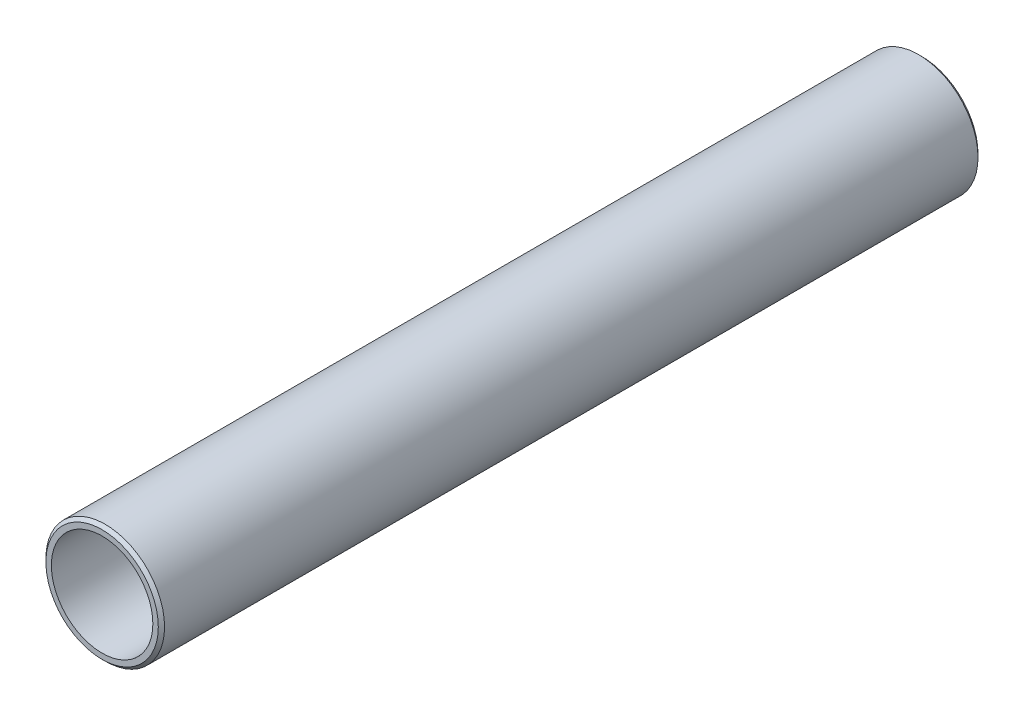
from build123d import *

# Parameters (mm, degrees)
SKETCH_1_R      = 38
SKETCH_1_R_2    = 32.5
EXTRUDE_1_DEPTH = 525
CHAMFER_1_SIZE  = 2


with BuildPart() as part:
    # 草图1 → 凸台-拉伸1 (new body)
    with BuildSketch(Plane.XY):
        Circle(SKETCH_1_R)
        Circle(SKETCH_1_R_2, mode=Mode.SUBTRACT)
    extrude(amount=EXTRUDE_1_DEPTH)

    # 倒角1
    chamfer_1_edges = [part.edges().sort_by_distance(p)[0] for p in [
        (-38, 0, 0),
        (-38, 0, 525),
    ]]
    chamfer(chamfer_1_edges, length=CHAMFER_1_SIZE)


solid = part.part
